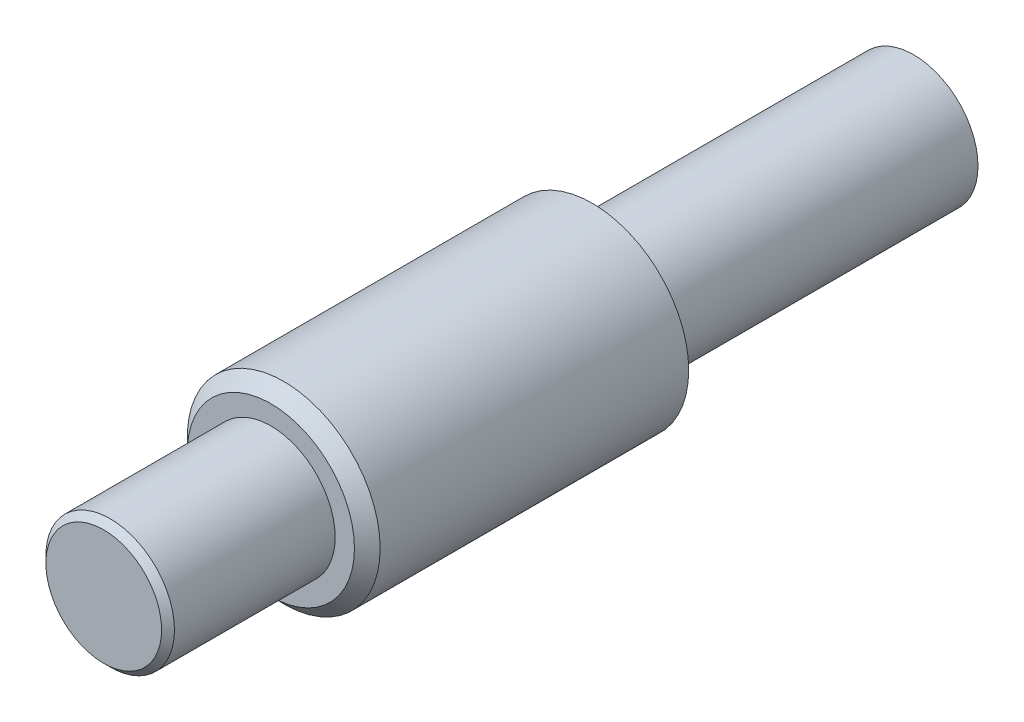
SolidWorks part; units mm, degrees
ref_plane "Front Plane" through (0, 0, 0) normal (0, 0, 1) x (1, 0, 0)
ref_plane "Top Plane" through (0, 0, 0) normal (0, 1, 0) x (1, 0, 0)
ref_plane "Right Plane" through (0, 0, 0) normal (1, 0, 0) x (0, 0, -1)
sketch "Sketch1" plane through (0, 0, 0) normal (0, 0, 1) x (1, 0, 0)
  circle A0 centre (0, 0) radius 5
  dimension "D1" = 10
extrude "Boss-Extrude1" add sketch "Sketch1" along normal blind 25
sketch "Sketch2" plane through (0, 0, 25) normal (0, 0, 1) x (1, 0, 0)
  circle A0 centre (0, 0) radius 7.5
  dimension "D1" = 15
extrude "Boss-Extrude2" add sketch "Sketch2" along normal blind 8
sketch "Sketch3" plane through (0, 0, 33) normal (0, 0, 1) x (1, 0, 0)
  circle A0 centre (0, 0) radius 5
  dimension "D1" = 10
extrude "Boss-Extrude3" add sketch "Sketch3" along normal blind 30
sketch "Sketch4" plane through (0, 0, 33) normal (0, 0, 1) x (1, 0, 0)
  circle A0 centre (0, 0) radius 7.5
extrude "Boss-Extrude4" add sketch "Sketch4" along normal blind 17
chamfer "Chamfer1" distance 1 angle 45 1 edges at (7.5, 0, 50)
chamfer "Chamfer2" distance 0.5 angle 45 1 edges at (5, 0, 63)
